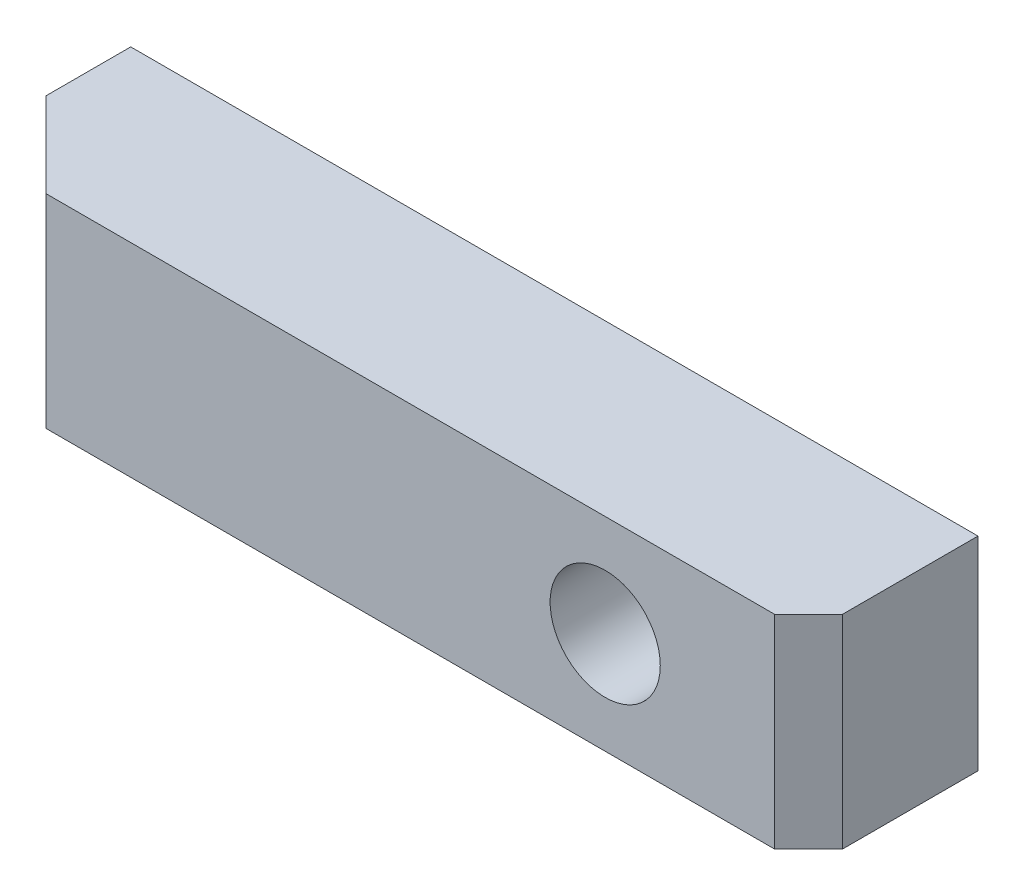
SolidWorks part; units mm, degrees
material "1023 碳钢板 (SS)"
ref_plane "Front Plane" through (0, 0, 0) normal (0, 0, 1) x (1, 0, 0)
ref_plane "Top Plane" through (0, 0, 0) normal (0, 1, 0) x (1, 0, 0)
ref_plane "Right Plane" through (0, 0, 0) normal (1, 0, 0) x (0, 0, -1)
ref_plane "Plane4" through (0, 6, 0) normal (0, 1, 0) x (1, 0, 0)
sketch "Sketch1" plane through (0, 6, 0) normal (0, 1, 0) x (1, 0, 0)
  line L0 (-20, -5) -> (25, -5)
  line L1 (25, -5) -> (25, 5)
  line L2 (25, 5) -> (-25, 5)
  line L3 (-25, 5) -> (-25, 0)
  line L4 (-25, 0) -> (-20, -5)
extrude "Boss-Extrude1" add sketch "Sketch1" against normal blind 12
hole_wizard "Ø6.5 (6.5) Diameter Hole1" positions "Sketch3" profile "Sketch2" hole size "Ø6.5" standard "ANSI Metric" end condition through all
sketch "Sketch3" plane through (0, 0, 5) normal (0, 0, 1) x (1, 0, 0)
  point P0 (13, 0)
sketch "Sketch2" plane through (13, 0, 5) normal (1, 0, 0) x (0, -1, 0)
  line L0 (0, 0) -> (0, 10)
  line L1 (0, 10) -> (3.25, 10)
  line L2 (3.25, 10) -> (3.25, 0)
  line L5 (3.25, 0) -> (0, 0)
  line L11 (0, -6.35) -> (0, 107.95) construction
  dimension "通孔孔直径" = 6.5
  dimension "通孔孔深度" = 10
chamfer "Chamfer1" distance 2 angle 45 1 edges at (25, 0, 5)
